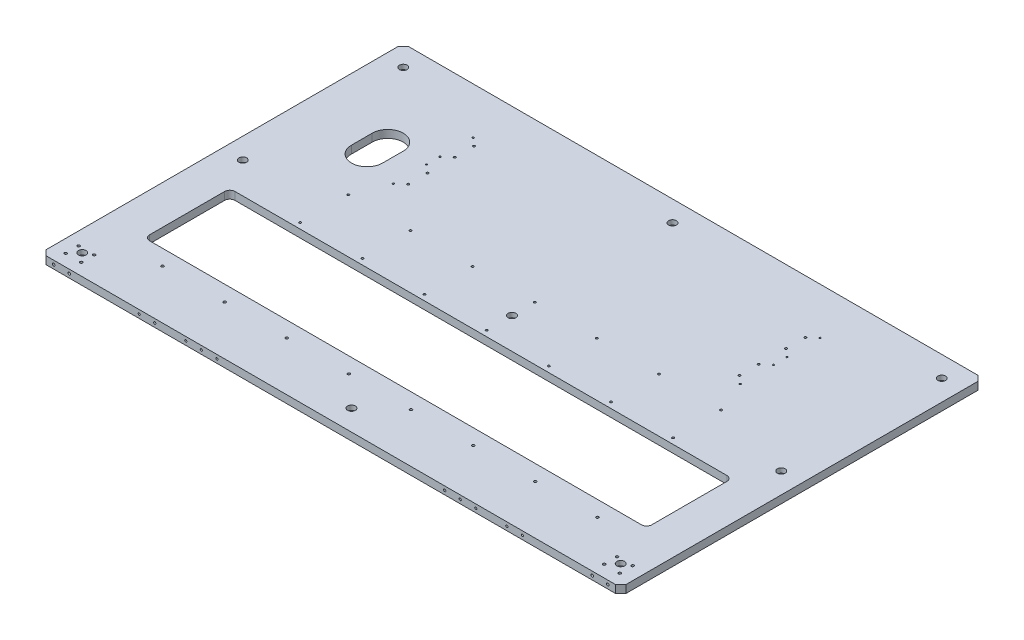
from build123d import *

# Parameters (mm, degrees)
SKETCH_1_W                = 1120
SKETCH_1_H                = 700
EXTRUDE_1_DEPTH           = 15
CHAMFER_1_SIZE            = 10
SKETCH_2_W                = 970
SKETCH_2_H                = 165
CUT_EXTRUDE_1_DEPTH       = 20
FILLET_1_R                = 10
HOLE_WIZARD_1_D           = 9
HOLE_WIZARD_1_DEPTH       = 19.75
HOLE_WIZARD_1_CBORE_D     = 15
HOLE_WIZARD_1_CBORE_DEPTH = 9
HOLE_WIZARD_1_TIP         = 2.703872786
HOLE_WIZARD_M6_1_D        = 5
HOLE_WIZARD_M6_1_DEPTH    = 15
HOLE_WIZARD_M6_1_TIP      = 1.502151548
HOLE_WIZARD_M5_1_D        = 4.2
HOLE_WIZARD_M5_1_DEPTH    = 20
HOLE_WIZARD_M5_1_TIP      = 1.2618073
CUT_EXTRUDE_2_DEPTH       = 20
HOLE_WIZARD_M5_2_D        = 4.2
HOLE_WIZARD_M5_2_DEPTH    = 20
HOLE_WIZARD_M5_2_TIP      = 1.2618073
HOLE_WIZARD_M4_1_D        = 3.3
HOLE_WIZARD_M4_1_DEPTH    = 20
HOLE_WIZARD_M4_1_TIP      = 0.991420021
HOLE_WIZARD_M5_3_D        = 4.2
HOLE_WIZARD_M5_3_DEPTH    = 20
HOLE_WIZARD_M5_3_TIP      = 1.2618073
HOLE_WIZARD_M5_4_D        = 4.2
HOLE_WIZARD_M5_4_DEPTH    = 12.4
HOLE_WIZARD_M5_4_TIP      = 1.2618073
HOLE_WIZARD_2_D           = 9
HOLE_WIZARD_2_DEPTH       = 19.75
HOLE_WIZARD_2_CBORE_D     = 15
HOLE_WIZARD_2_CBORE_DEPTH = 9
HOLE_WIZARD_2_TIP         = 2.703872786
HOLE_WIZARD_M6_2_D        = 5
HOLE_WIZARD_M6_2_DEPTH    = 15
HOLE_WIZARD_M6_2_TIP      = 1.502151548
HOLE_WIZARD_M6_3_D        = 5
HOLE_WIZARD_M6_3_DEPTH    = 15
HOLE_WIZARD_M6_3_TIP      = 1.502151548


with BuildPart() as part:
    # 草图1 → 凸台-拉伸1 (new body)
    with BuildSketch(Plane(origin=(0, 0, 0), x_dir=(1, 0, 0), z_dir=(0, 1, 0))):
        Rectangle(SKETCH_1_W, SKETCH_1_H)
    extrude(amount=EXTRUDE_1_DEPTH)

    # 倒角1
    chamfer_1_edges = [part.edges().sort_by_distance(p)[0] for p in [
        (560, 7.5, 350),
        (-560, 7.5, 350),
        (-560, 7.5, -350),
        (560, 7.5, -350),
    ]]
    chamfer(chamfer_1_edges, length=CHAMFER_1_SIZE)

    # 草图2 → 切除-拉伸1 (cut)
    with BuildSketch(Plane(origin=(0, 15, 0), x_dir=(1, 0, 0), z_dir=(0, 1, 0))):
        with Locations((0, -142.5)):
            Rectangle(SKETCH_2_W, SKETCH_2_H)
    extrude(amount=-CUT_EXTRUDE_1_DEPTH, mode=Mode.SUBTRACT)

    # 圆角1
    fillet_1_edges = [part.edges().sort_by_distance(p)[0] for p in [
        (485, 7.5, 60),
        (485, 7.5, 225),
        (-485, 7.5, 225),
        (-485, 7.5, 60),
    ]]
    fillet(fillet_1_edges, radius=FILLET_1_R)

    # 打孔尺寸(%根据)内六角圆柱头螺钉的类型1
    with Locations(Plane(origin=(0, 15, 0), x_dir=(1, 0, 0), z_dir=(0, 1, 0))):
        with Locations((520, -310), (520, 0), (520, 310), (-520, -310), (-520, 0), (-520, 310)):
            CounterBoreHole(HOLE_WIZARD_1_D / 2, HOLE_WIZARD_1_CBORE_D / 2, HOLE_WIZARD_1_CBORE_DEPTH, depth=HOLE_WIZARD_1_DEPTH)
            with Locations((0, 0, -(HOLE_WIZARD_1_DEPTH + HOLE_WIZARD_1_TIP / 2))):  # 118° drill point
                Cone(0, HOLE_WIZARD_1_D / 2, HOLE_WIZARD_1_TIP, mode=Mode.SUBTRACT)

    # M6 螺纹孔1
    with Locations(Plane(origin=(0, 15, 0), x_dir=(1, 0, 0), z_dir=(0, 1, 0))):
        with Locations((-420, -255), (-300, -255), (-180, -255), (-60, -255), (60, -255), (180, -255), (300, -255), (420, -255)):
            Hole(HOLE_WIZARD_M6_1_D / 2, depth=HOLE_WIZARD_M6_1_DEPTH)
            with Locations((0, 0, -(HOLE_WIZARD_M6_1_DEPTH + HOLE_WIZARD_M6_1_TIP / 2))):  # 118° drill point
                Cone(0, HOLE_WIZARD_M6_1_D / 2, HOLE_WIZARD_M6_1_TIP, mode=Mode.SUBTRACT)

    # M5 螺纹孔1
    with Locations(Plane(origin=(0, 15, 0), x_dir=(1, 0, 0), z_dir=(0, 1, 0))):
        with Locations((360, -49), (360, 44), (240, -49), (240, 44), (120, -49), (120, 44), (0, -49), (0, 44), (-120, -49), (-120, 44), (-240, -49), (-240, 44), (-360, -49), (-360, 44)):
            Hole(HOLE_WIZARD_M5_1_D / 2, depth=HOLE_WIZARD_M5_1_DEPTH)
            with Locations((0, 0, -(HOLE_WIZARD_M5_1_DEPTH + HOLE_WIZARD_M5_1_TIP / 2))):  # 118° drill point
                Cone(0, HOLE_WIZARD_M5_1_D / 2, HOLE_WIZARD_M5_1_TIP, mode=Mode.SUBTRACT)

    # 草图9 → 切除-拉伸2 (cut)
    with BuildSketch(Plane(origin=(0, 15, 0), x_dir=(1, 0, 0), z_dir=(0, 1, 0))):
        with BuildLine():
            Line((-440, 130), (-440, 170))
            ThreePointArc((-440, 170), (-410, 200), (-380, 170))
            Line((-380, 170), (-380, 130))
            ThreePointArc((-380, 130), (-410, 100), (-440, 130))
        make_face()
    extrude(amount=-CUT_EXTRUDE_2_DEPTH, mode=Mode.SUBTRACT)

    # M5 螺纹孔2
    with Locations(Plane.XY.offset(350)):
        with Locations((-280, 7.5), (-250, 7.5), (-220, 7.5), (280, 7.5), (250, 7.5), (220, 7.5)):
            Hole(HOLE_WIZARD_M5_2_D / 2, depth=HOLE_WIZARD_M5_2_DEPTH)
            with Locations((0, 0, -(HOLE_WIZARD_M5_2_DEPTH + HOLE_WIZARD_M5_2_TIP / 2))):  # 118° drill point
                Cone(0, HOLE_WIZARD_M5_2_D / 2, HOLE_WIZARD_M5_2_TIP, mode=Mode.SUBTRACT)

    # M4 螺纹孔1
    with Locations(Plane(origin=(0, 15, 0), x_dir=(1, 0, 0), z_dir=(0, 1, 0))):
        with Locations((335, 106), (335, 170), (-335, 106), (-335, 170), (-335, 196), (-335, 260), (335, 196), (335, 260)):
            Hole(HOLE_WIZARD_M4_1_D / 2, depth=HOLE_WIZARD_M4_1_DEPTH)
            with Locations((0, 0, -(HOLE_WIZARD_M4_1_DEPTH + HOLE_WIZARD_M4_1_TIP / 2))):  # 118° drill point
                Cone(0, HOLE_WIZARD_M4_1_D / 2, HOLE_WIZARD_M4_1_TIP, mode=Mode.SUBTRACT)

    # M5 螺纹孔3
    with Locations(Plane(origin=(0, 15, 0), x_dir=(1, 0, 0), z_dir=(0, 1, 0))):
        with Locations((320, 119.5), (320, 156.5), (320, 209.5), (320, 246.5), (-320, 119.5), (-320, 156.5), (-320, 209.5), (-320, 246.5)):
            Hole(HOLE_WIZARD_M5_3_D / 2, depth=HOLE_WIZARD_M5_3_DEPTH)
            with Locations((0, 0, -(HOLE_WIZARD_M5_3_DEPTH + HOLE_WIZARD_M5_3_TIP / 2))):  # 118° drill point
                Cone(0, HOLE_WIZARD_M5_3_D / 2, HOLE_WIZARD_M5_3_TIP, mode=Mode.SUBTRACT)

    # M5 螺纹孔4
    with Locations(Plane.XY.offset(350)):
        with Locations((-370, 7.5), (-340, 7.5), (370, 7.5), (340, 7.5)):
            Hole(HOLE_WIZARD_M5_4_D / 2, depth=HOLE_WIZARD_M5_4_DEPTH)
            with Locations((0, 0, -(HOLE_WIZARD_M5_4_DEPTH + HOLE_WIZARD_M5_4_TIP / 2))):  # 118° drill point
                Cone(0, HOLE_WIZARD_M5_4_D / 2, HOLE_WIZARD_M5_4_TIP, mode=Mode.SUBTRACT)

    # 打孔尺寸(%根据)内六角圆柱头螺钉的类型2
    with Locations(Plane(origin=(0, 15, 0), x_dir=(1, 0, 0), z_dir=(0, 1, 0))):
        with Locations((0, 310), (0, 0), (0, -310)):
            CounterBoreHole(HOLE_WIZARD_2_D / 2, HOLE_WIZARD_2_CBORE_D / 2, HOLE_WIZARD_2_CBORE_DEPTH, depth=HOLE_WIZARD_2_DEPTH)
            with Locations((0, 0, -(HOLE_WIZARD_2_DEPTH + HOLE_WIZARD_2_TIP / 2))):  # 118° drill point
                Cone(0, HOLE_WIZARD_2_D / 2, HOLE_WIZARD_2_TIP, mode=Mode.SUBTRACT)

    # M6 螺纹孔2
    with Locations(Plane.XY.offset(350)):
        with Locations((-535, 7.5), (-505, 7.5), (505, 7.5), (535, 7.5)):
            Hole(HOLE_WIZARD_M6_2_D / 2, depth=HOLE_WIZARD_M6_2_DEPTH)
            with Locations((0, 0, -(HOLE_WIZARD_M6_2_DEPTH + HOLE_WIZARD_M6_2_TIP / 2))):  # 118° drill point
                Cone(0, HOLE_WIZARD_M6_2_D / 2, HOLE_WIZARD_M6_2_TIP, mode=Mode.SUBTRACT)

    # M6 螺纹孔3
    with Locations(Plane(origin=(0, 15, 0), x_dir=(1, 0, 0), z_dir=(0, 1, 0))):
        with Locations((535, -327), (505, -327), (535, -302), (505, -302), (-505, -327), (-535, -327), (-505, -302), (-535, -302)):
            Hole(HOLE_WIZARD_M6_3_D / 2, depth=HOLE_WIZARD_M6_3_DEPTH)
            with Locations((0, 0, -(HOLE_WIZARD_M6_3_DEPTH + HOLE_WIZARD_M6_3_TIP / 2))):  # 118° drill point
                Cone(0, HOLE_WIZARD_M6_3_D / 2, HOLE_WIZARD_M6_3_TIP, mode=Mode.SUBTRACT)


solid = part.part
